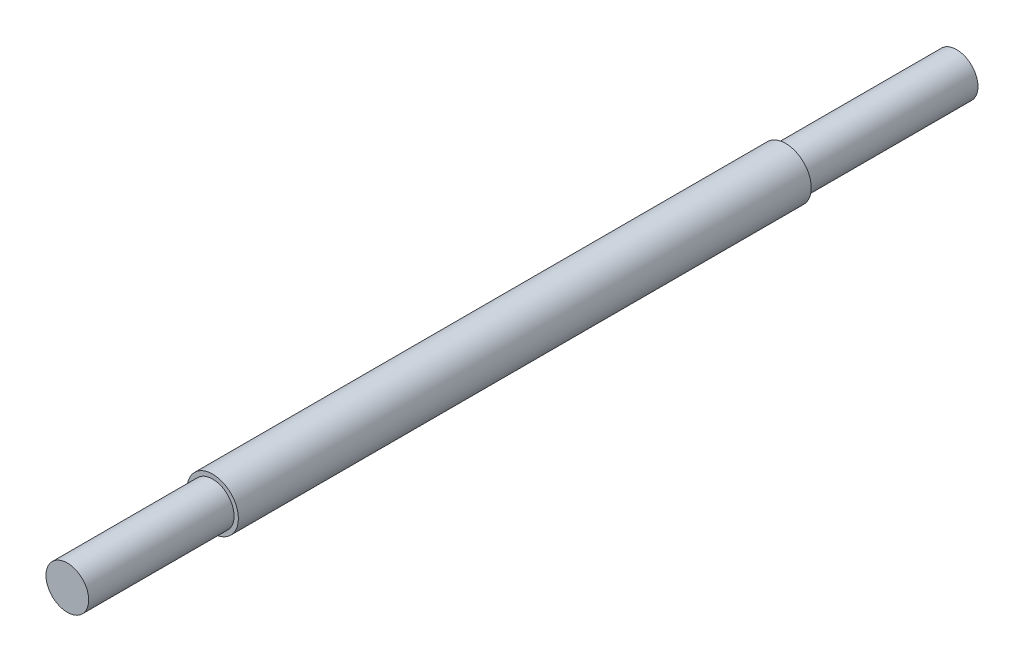
from build123d import *

# Parameters (mm, degrees)
SKETCH1_R           = 2.5
BOSS_EXTRUDE1_DEPTH = 20
SKETCH2_R           = 3
BOSS_EXTRUDE2_DEPTH = 67
SKETCH3_R           = 2.5
BOSS_EXTRUDE3_DEPTH = 17


with BuildPart() as part:
    # Sketch1 → Boss-Extrude1 (new body)
    with BuildSketch(Plane.XY):
        Circle(SKETCH1_R)
    extrude(amount=BOSS_EXTRUDE1_DEPTH)

    # Sketch2 → Boss-Extrude2 (add)
    with BuildSketch(Plane.XY.offset(20)):
        Circle(SKETCH2_R)
    extrude(amount=BOSS_EXTRUDE2_DEPTH)

    # Sketch3 → Boss-Extrude3 (add)
    with BuildSketch(Plane.XY.offset(87)):
        Circle(SKETCH3_R)
    extrude(amount=BOSS_EXTRUDE3_DEPTH)


solid = part.part
